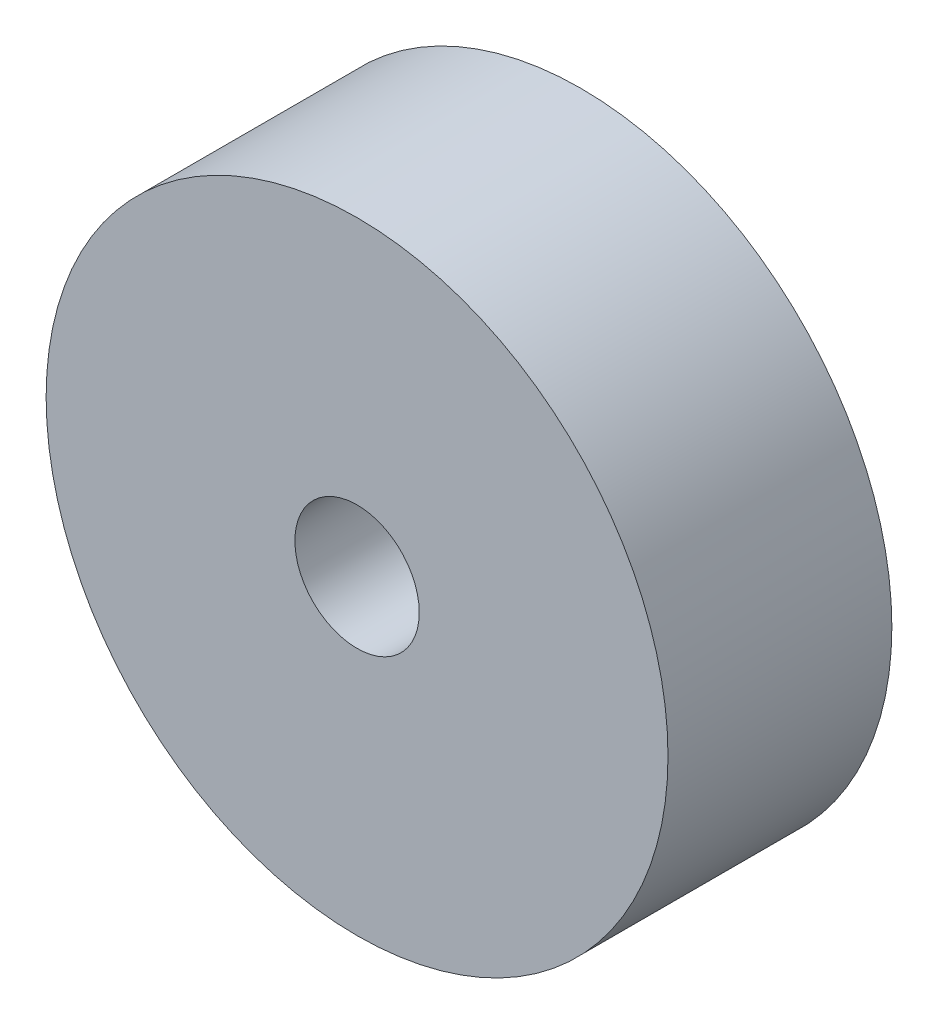
from build123d import *

# Parameters (mm, degrees)
SKETCH_1_W = 10
SKETCH_1_H = 9


with BuildPart() as part:
    # 草图1 → 旋转1 (revolve)
    with BuildSketch(Plane(origin=(0, 0, 0), x_dir=(1, 0, 0), z_dir=(0, 1, 0)), mode=Mode.PRIVATE) as revolve_1_sk:
        with Locations((-7.5, 4.5)):
            Rectangle(SKETCH_1_W, SKETCH_1_H)
    revolve(revolve_1_sk.sketch.rotate(Axis((0, 0, 129.063142874), (0, 0, -1)), 180), axis=Axis((0, 0, 129.063142874), (0, 0, -1)))


solid = part.part
